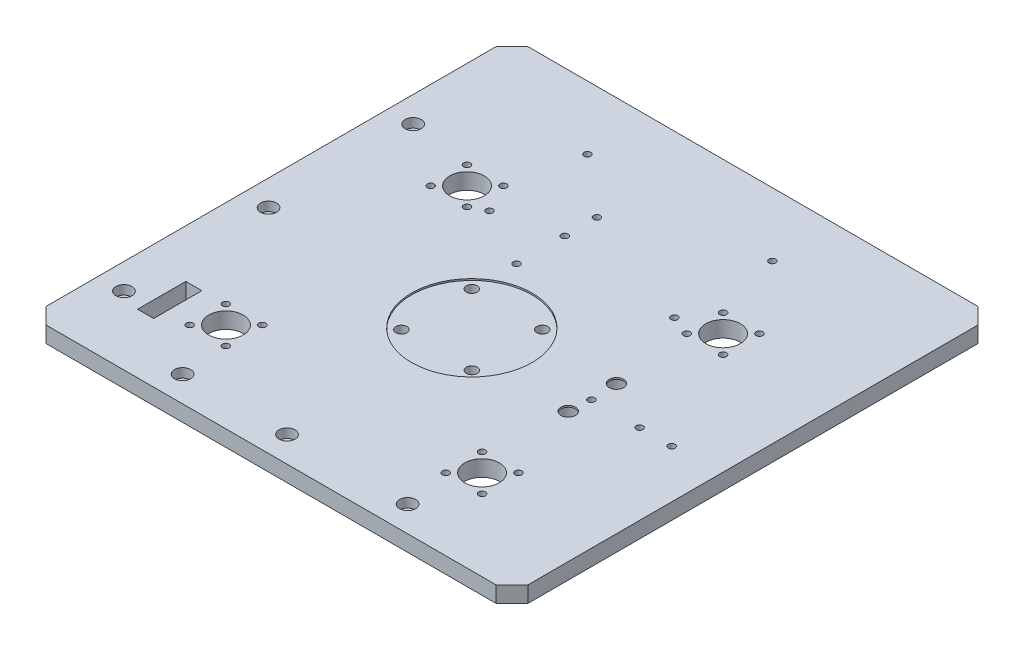
SolidWorks part; units mm, degrees
ref_plane "Front Plane" through (0, 0, 0) normal (0, 0, 1) x (1, 0, 0)
ref_plane "Top Plane" through (0, 0, 0) normal (0, 1, 0) x (1, 0, 0)
ref_plane "Right Plane" through (0, 0, 0) normal (1, 0, 0) x (0, 0, -1)
sketch "Sketch1" plane through (0, 0, 0) normal (0, 1, 0) x (1, 0, 0)
  line L1 (-150, -150) -> (150, -150)
  line L2 (-150, -150) -> (-150, 150)
  line L3 (-150, 150) -> (150, 150)
  line L4 (150, -150) -> (150, 150)
  line L5 (-150, -150) -> (150, 150) construction
  line L6 (-150, 150) -> (150, -150) construction
  point P0 (0, 0)
  dimension "D1" = 300
  dimension "D2" = 300
extrude "Boss-Extrude1" add sketch "Sketch1" along normal blind 10
sketch "Sketch2" plane through (0, 10, 0) normal (0, 1, 0) x (1, 0, 0)
  circle A0 centre (-6, -19) radius 37.5
  dimension "D1" = 75
extrude "Cut-Extrude1" cut sketch "Sketch2" against normal blind 1
sketch "Sketch3" plane through (0, 10, 0) normal (0, 1, 0) x (1, 0, 0)
  line L0 (114, -128) -> (-126, -128) construction
  line L1 (-110, -113) -> (-120, -113)
  line L2 (-110, -113) -> (-110, -83)
  line L3 (-110, -83) -> (-120, -83)
  line L4 (-120, -113) -> (-120, -83)
  line L5 (-128, 105) -> (-128, -140) construction
  dimension "D1" = 10
  dimension "D2" = 30
  dimension "D3" = 15
  dimension "D4" = 8
extrude "Cut-Extrude2" cut sketch "Sketch3" against normal through all
sketch "Sketch4" plane through (0, 10, 0) normal (0, 1, 0) x (1, 0, 0)
  circle A0 centre (-84, -94) radius 10.75
  circle A1 centre (-84, 56) radius 10.75
  circle A2 centre (75.3603, 56) radius 10.75
  circle A3 centre (75.3603, -94) radius 10.75
  dimension "D1" = 21.5
extrude "Cut-Extrude3" cut sketch "Sketch4" against normal through all
hole_wizard "CBORE for M8 Hexagon socket head cap screws1" positions "Sketch5" profile "Sketch6" counterbore size "M8" standard "GB" end condition through all
sketch "Sketch5" plane through (0, 0, 0) normal (0, -1, 0) x (-1, 0, 0)
  point P0 (-69, -4)
  point P3 (-69, -34)
sketch "Sketch6" plane through (69, 0, 4) normal (1, 0, 0) x (0, 0, -1)
  line L0 (0, 0) -> (0, 10)
  line L1 (0, 10) -> (4.5, 10)
  line L3 (4.5, 10) -> (4.5, 9)
  line L4 (4.5, 9) -> (7.5, 9)
  line L5 (7.5, 9) -> (7.5, 0)
  line L7 (7.5, 0) -> (0, 0)
  line L11 (0, -6.35) -> (0, 107.95) construction
  dimension "通孔孔直径" = 9
  dimension "通孔孔深度" = 10
  dimension "柱形沉头孔直径" = 15
  dimension "柱形沉头孔深度" = 9
hole_wizard "M8 Tapped Hole1" positions "Sketch9" profile "Sketch10" tap size "M8" standard "GB" end condition through all
sketch "Sketch9" plane through (0, 10, 0) normal (0, 1, 0) x (1, 0, 0)
  point P0 (15.9222, -40.9184)
  point P3 (15.9184, 2.9222)
  point P6 (-27.9222, 2.9184)
  point P9 (-27.9184, -40.9222)
sketch "Sketch10" plane through (15.9222, 10, 40.9184) normal (1, 0, 0) x (0, 0, 1)
  line L0 (0, 0) -> (0, 10)
  line L1 (0, 10) -> (3.4, 10)
  line L2 (3.4, 10) -> (3.4, 0)
  line L5 (3.4, 0) -> (0, 0)
  line L11 (0, -6.35) -> (0, 107.95) construction
  dimension "通孔螺纹孔钻头直径" = 6.8
  dimension "通孔螺纹孔钻头深度" = 10
cosmetic thread "Hole thread line1" parameters "D2"=8
cosmetic thread "Hole thread line2" parameters "D2"=8
cosmetic thread "Hole thread line3" parameters "D2"=8
cosmetic thread "Hole thread line4" parameters "D2"=8
hole_wizard "M5 Tapped Hole1" positions "Sketch11" profile "Sketch12" tap size "M5" standard "GB" end condition through all
sketch "Sketch11" plane through (0, 0, 0) normal (0, -1, 0) x (-1, 0, 0)
  point P0 (72.6863, 44.6863)
  point P3 (95.3137, 44.6863)
  point P6 (95.3137, 67.3137)
  point P9 (72.6863, 67.3137)
  point P11 (95.3137, -82.6863)
  point P14 (95.3137, -105.3137)
  point P17 (72.6863, -105.3137)
  point P20 (72.6863, -82.6863)
  point P23 (-64.0466, -82.6863)
  point P26 (-64.0466, -105.3137)
  point P29 (-86.674, -105.3137)
  point P32 (-86.674, -82.6863)
  point P35 (-64.0466, 67.3137)
  point P38 (-64.0466, 44.6863)
  point P41 (-86.674, 44.6863)
  point P44 (-86.674, 67.3137)
sketch "Sketch12" plane through (-72.6863, 0, -44.6863) normal (1, 0, 0) x (0, 0, -1)
  line L0 (0, 0) -> (0, 10)
  line L1 (0, 10) -> (2.1, 10)
  line L2 (2.1, 10) -> (2.1, 0)
  line L5 (2.1, 0) -> (0, 0)
  line L11 (0, -6.35) -> (0, 107.95) construction
  dimension "通孔螺纹孔钻头直径" = 4.2
  dimension "通孔螺纹孔钻头深度" = 10
cosmetic thread "Hole thread line5" parameters "D2"=5
cosmetic thread "Hole thread line6" parameters "D2"=5
cosmetic thread "Hole thread line7" parameters "D2"=5
cosmetic thread "Hole thread line8" parameters "D2"=5
cosmetic thread "Hole thread line9" parameters "D2"=5
cosmetic thread "Hole thread line10" parameters "D2"=5
cosmetic thread "Hole thread line11" parameters "D2"=5
cosmetic thread "Hole thread line12" parameters "D2"=5
cosmetic thread "Hole thread line13" parameters "D2"=5
cosmetic thread "Hole thread line14" parameters "D2"=5
cosmetic thread "Hole thread line15" parameters "D2"=5
cosmetic thread "Hole thread line16" parameters "D2"=5
cosmetic thread "Hole thread line17" parameters "D2"=5
cosmetic thread "Hole thread line18" parameters "D2"=5
cosmetic thread "Hole thread line19" parameters "D2"=5
cosmetic thread "Hole thread line20" parameters "D2"=5
hole_wizard "M5 Tapped Hole2" positions "Sketch13" profile "Sketch14" tap size "M5" standard "GB" end condition through all
sketch "Sketch13" plane through (0, 10, 0) normal (0, 1, 0) x (1, 0, 0)
  line L0 (-60.55, 110.5) -> (-70.8948, 110.5) construction
  line L1 (-60.55, 103) -> (-60.55, 118) construction
  line L3 (-73.5, 80) -> (61.5, 80) construction
  line L4 (-73.5, 35) -> (-73.5, 125) construction
  line L5 (61.5, 35) -> (61.5, 125) construction
  line L7 (-6, 130) -> (-6, 30) construction
  line L8 (-51.4, 130) -> (39.4, 130) construction
  line L9 (-51.4, 30) -> (39.4, 30) construction
  line L10 (-66.55, 118) -> (-66.55, 103) construction
  line L11 (-60.55, 49.5) -> (-70.8948, 49.5) construction
  line L12 (48.55, 49.5) -> (58.8948, 49.5) construction
  line L13 (48.55, 110.5) -> (58.8948, 110.5) construction
  point P23 (-63.55, 110.5)
  point P30 (-63.55, 49.5)
  point P35 (51.55, 49.5)
  point P36 (51.55, 110.5)
  dimension "D1" = 3
sketch "Sketch14" plane through (51.55, 10, -110.5) normal (1, 0, 0) x (0, 0, 1)
  line L0 (0, 0) -> (0, 10)
  line L1 (0, 10) -> (2.1, 10)
  line L2 (2.1, 10) -> (2.1, 0)
  line L5 (2.1, 0) -> (0, 0)
  line L11 (0, -6.35) -> (0, 107.95) construction
  dimension "通孔螺纹孔钻头直径" = 4.2
  dimension "通孔螺纹孔钻头深度" = 10
cosmetic thread "Hole thread line21" parameters "D2"=5
cosmetic thread "Hole thread line22" parameters "D2"=5
cosmetic thread "Hole thread line23" parameters "D2"=5
cosmetic thread "Hole thread line24" parameters "D2"=5
chamfer "Chamfer1" distance 10 angle 45 4 edges at (-150, 5, 150) (150, 5, 150) (150, 5, -150) (-150, 5, -150)
hole_wizard "M5 Tapped Hole3" positions "Sketch15" profile "Sketch16" tap size "M5" standard "GB"
sketch "Sketch15" plane through (0, 0, 0) normal (0, -1, 0) x (-1, 0, 0)
  point P0 (26.5781, 59.4136)
  point P3 (-100, -20.593)
  point P7 (26.5781, 79.4136)
  point P9 (26.5781, 29.4136)
  point P11 (-120, -20.593)
  point P13 (-70, -20.593)
  dimension "D1" = 30
  dimension "D2" = 20
  dimension "D3" = 20
  dimension "D4" = 30
sketch "Sketch16" plane through (-26.5781, 0, -59.4136) normal (1, 0, 0) x (0, 0, -1)
  line L0 (0, 0) -> (0, 38.1618)
  line L1 (0, 38.1618) -> (2.1, 36.9)
  line L2 (2.1, 36.9) -> (2.1, 0)
  line L5 (2.1, 0) -> (0, 0)
  line L10 (0, 38.1618) -> (-2.1, 36.9) construction
  line L11 (0, -6.35) -> (0, 107.95) construction
  dimension "螺纹孔钻头直径" = 4.2
  dimension "螺纹孔钻头深度" = 36.9
  dimension "导头角度" = 118
cosmetic thread "Hole thread line25" parameters "D1"=32.9, "D2"=5
cosmetic thread "Hole thread line26" parameters "D1"=32.9, "D2"=5
cosmetic thread "Hole thread line27" parameters "D1"=32.9, "D2"=5
cosmetic thread "Hole thread line28" parameters "D1"=32.9, "D2"=5
cosmetic thread "Hole thread line29" parameters "D1"=32.9, "D2"=5
cosmetic thread "Hole thread line30" parameters "D1"=32.9, "D2"=5
hole_wizard "CBORE for M5 Hexagon socket head cap screws1" positions "Sketch17" profile "Sketch18" counterbore size "M5" standard "GB"
sketch "Sketch17" plane through (0, 10, 0) normal (0, 1, 0) x (1, 0, 0)
  line L0 (114, -134) -> (-126, -134) construction
  line L1 (114, -128) -> (114, -140) construction
  line L2 (-126, -128) -> (-126, -140) construction
  line L3 (-134, 105) -> (-134, -140) construction
  line L4 (-128, 105) -> (-140, 105) construction
  line L5 (-128, -140) -> (-140, -140) construction
  point P16 (-71, -134)
  point P18 (-6, -134)
  point P20 (69, -134)
  point P33 (-134, 72.5)
  point P35 (-134, -17.5)
  point P37 (-134, -107.5)
  dimension "D1" = 75
  dimension "D2" = 65
  dimension "D3" = 90
  dimension "D4" = 90
sketch "Sketch18" plane through (-134, 10, 107.5) normal (1, 0, 0) x (0, 0, 1)
  line L0 (0, 0) -> (0, 38.5524)
  line L1 (0, 38.5524) -> (2.75, 36.9)
  line L2 (2.75, 36.9) -> (2.75, 5.7)
  line L3 (2.75, 5.7) -> (5, 5.7)
  line L4 (5, 5.7) -> (5, 0)
  line L5 (5, 0) -> (0, 0)
  line L10 (0, 38.5524) -> (-2.75, 36.9) construction
  line L11 (0, -6.35) -> (0, 107.95) construction
  dimension "孔直径" = 5.5
  dimension "孔深度" = 36.9
  dimension "柱形沉头孔直径" = 10
  dimension "柱形沉头孔深度" = 5.7
  dimension "导头角度" = 118
equation "\"1\"= \"代号代号\""
equation "\"2\"= \"名称代号\""
